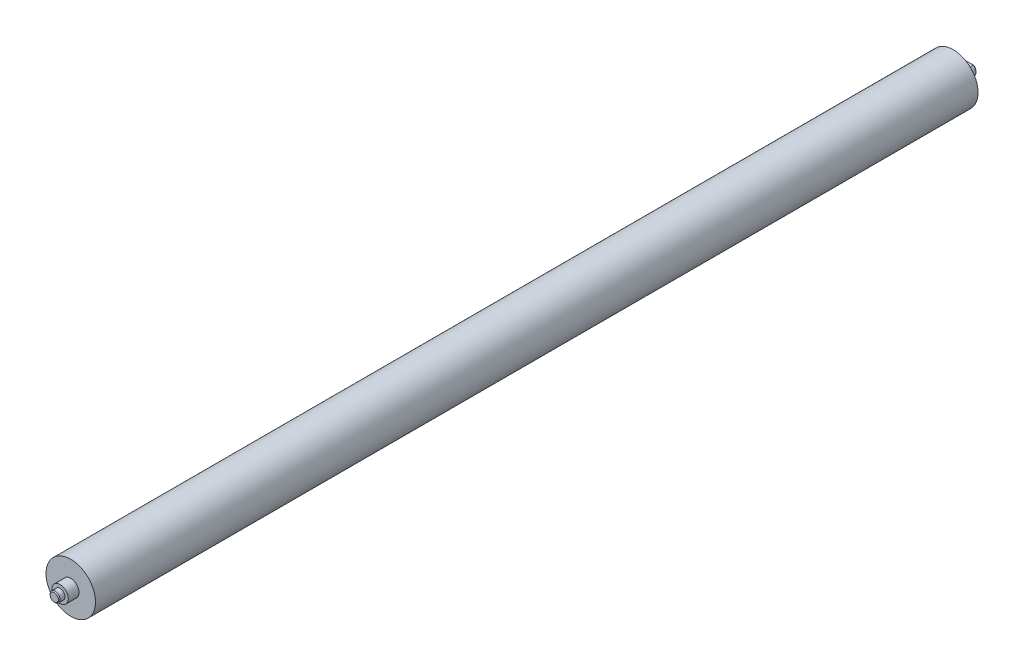
from build123d import *

# Parameters (mm, degrees)
SKETCH1_W           = 30
SKETCH1_H           = 1070
SKETCH2_R           = 10
BOSS_EXTRUDE1_DEPTH = 6
BOSS_EXTRUDE2_DEPTH = 15
BOSS_EXTRUDE3_START = 13
SKETCH4_R           = 10
BOSS_EXTRUDE3_DEPTH = 13
SKETCH5_R           = 6
BOSS_EXTRUDE4_DEPTH = 7
CHAMFER1_SIZE       = 1


with BuildPart() as part:
    # Sketch1 → Revolve1 (revolve)
    with BuildSketch(Plane.XZ, mode=Mode.PRIVATE) as revolve1_sk:
        with Locations((15, 0)):
            Rectangle(SKETCH1_W, SKETCH1_H)
    revolve(revolve1_sk.sketch.rotate(Axis((0, 0, 535), (0, 0, -1)), 180), axis=Axis((0, 0, 535), (0, 0, -1)))

    # Sketch2 → Boss-Extrude1 (add)
    with BuildSketch(Plane(origin=(0, 0, -535), x_dir=(-1, 0, 0), z_dir=(0, 0, -1))):
        Circle(SKETCH2_R)
    extrude(amount=BOSS_EXTRUDE1_DEPTH)

    # Sketch3 → Boss-Extrude2 (add)
    with BuildSketch(Plane(origin=(0, 0, -541), x_dir=(-1, 0, 0), z_dir=(0, 0, -1))):
        with BuildLine():
            Line((-4.5, 6), (4.5, 6))
            ThreePointArc((4.5, 6), (7.5, 0), (4.5, -6))
            Line((4.5, -6), (-4.5, -6))
            ThreePointArc((-4.5, -6), (-7.5, 0), (-4.5, 6))
        make_face()
    extrude(amount=BOSS_EXTRUDE2_DEPTH)

    # Sketch4 → Boss-Extrude3 (add)
    with BuildSketch(Plane.XY.offset(535).offset(BOSS_EXTRUDE3_START)):
        with Locations(Location((0, 0, 0), (0, 0, 180))):
            Circle(SKETCH4_R)
    extrude(amount=-BOSS_EXTRUDE3_DEPTH)

    # Sketch5 → Boss-Extrude4 (add)
    with BuildSketch(Plane.XY.offset(548)):
        with Locations(Location((0, 0, 0), (0, 0, 180))):
            Circle(SKETCH5_R)
    extrude(amount=BOSS_EXTRUDE4_DEPTH)

    # Chamfer1
    chamfer1_edges = [part.edges().sort_by_distance(p)[0] for p in [
        (7.5, 0, -556),
        (0, -6, -556),
        (-7.5, 0, -556),
        (0, 6, -556),
        (6, 0, 555),
    ]]
    chamfer(chamfer1_edges, length=CHAMFER1_SIZE)


solid = part.part
